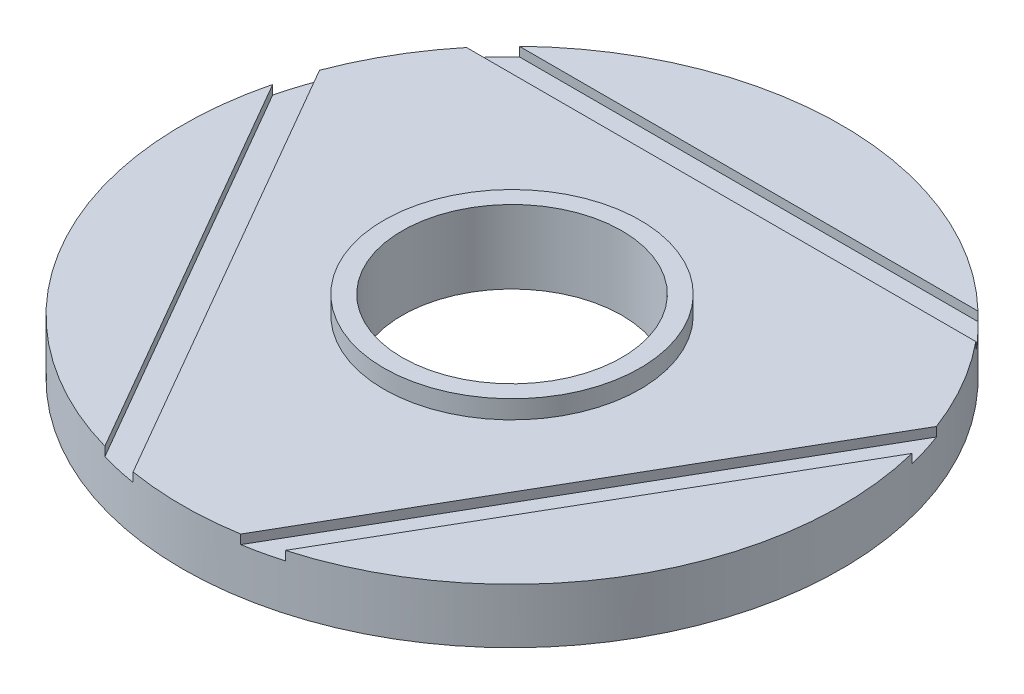
SolidWorks part; units mm, degrees
ref_plane "Front Plane" through (0, 0, 0) normal (0, 0, 1) x (1, 0, 0)
ref_plane "Top Plane" through (0, 0, 0) normal (0, 1, 0) x (1, 0, 0)
ref_plane "Right Plane" through (0, 0, 0) normal (1, 0, 0) x (0, 0, -1)
sketch "Sketch1" plane through (0, 0, 0) normal (0, 1, 0) x (1, 0, 0)
  circle A0 centre (0, 0) radius 180
  circle A1 centre (0, 0) radius 60
  dimension "D1" = 360
  dimension "D2" = 120
extrude "Boss-Extrude1" add sketch "Sketch1" along normal blind 30
sketch "Sketch2" plane through (0, 30, 0) normal (0, 1, 0) x (1, 0, 0)
  circle A0 centre (0, 0) radius 60
  circle A1 centre (0, 0) radius 70
extrude "Boss-Extrude2" add sketch "Sketch2" along normal blind 10
sketch "Sketch4" plane through (0, 30, 0) normal (0, 1, 0) x (1, 0, 0)
  line L0 (-186.6117, 114.25) -> (200.6752, 114.25)
  line L1 (200.6752, 114.25) -> (200.6752, 129.25)
  line L2 (200.6752, 129.25) -> (-186.6117, 129.25)
  line L3 (-186.6117, 129.25) -> (-186.6117, 114.25)
  dimension "D1" = 114.25
  dimension "D2" = 15
extrude "Cut-Extrude2" cut sketch "Sketch4" against normal blind 5
pattern_circular "CirPattern1" count 3 over 360 about axis through (0, 0, 0) along (0, 1, 0) of "Cut-Extrude2"
